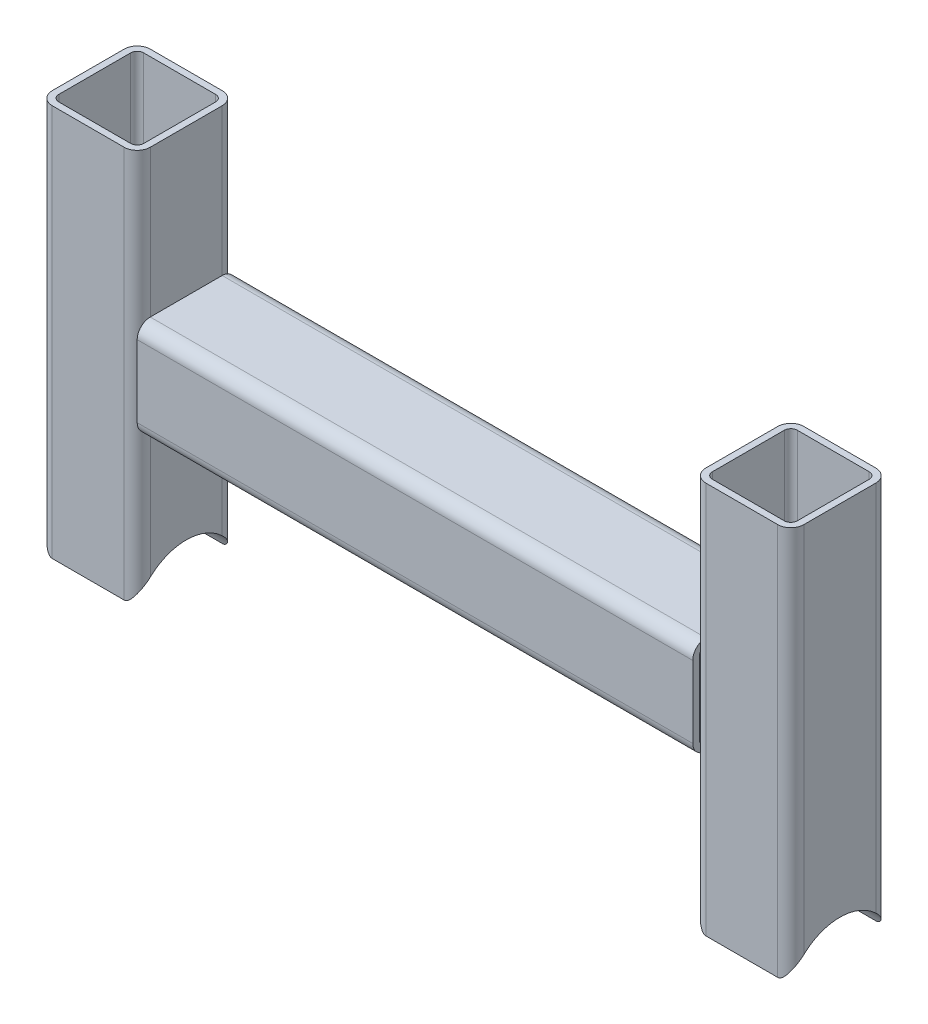
from build123d import *

# Parameters (mm, degrees)
GB_T_6728_2002_SQUARE_HOLLOW_SECTION_STE_DEPTH = 120
GB_T_6728_2002_SQUARE_HOLLOW_SECTION_2_DEPTH   = 120
GB_T_6728_2002_SQUARE_HOLLOW_SECTION_3_DEPTH   = 202
CUT_EXTRUDE1_DEPTH                             = 131.575648572
CUT_EXTRUDE1_DEPTH_BACK                        = 131.575648572
SKETCH3_R                                      = 16


with BuildPart() as part:
    # Sketch1 → Gb／t 6728—2002 Square hollow section steel 30×2-example.com(1) (new body)
    with BuildSketch(Plane(origin=(-100, -60, 0), x_dir=(-1, 0, 0), z_dir=(0, 1, 0))):
        with BuildLine():
            Line((-11, -15), (11, -15))
            ThreePointArc((11, -15), (13.828427125, -13.828427125), (15, -11))
            Line((15, -11), (15, 11))
            ThreePointArc((15, 11), (13.828427125, 13.828427125), (11, 15))
            Line((11, 15), (-11, 15))
            ThreePointArc((-11, 15), (-13.828427125, 13.828427125), (-15, 11))
            Line((-15, 11), (-15, -11))
            ThreePointArc((-15, -11), (-13.828427125, -13.828427125), (-11, -15))
        make_face()
        with BuildLine():
            Line((-11, -13), (11, -13))
            ThreePointArc((11, -13), (12.414213562, -12.414213562), (13, -11))
            Line((13, -11), (13, 11))
            ThreePointArc((13, 11), (12.414213562, 12.414213562), (11, 13))
            Line((11, 13), (-11, 13))
            ThreePointArc((-11, 13), (-12.414213562, 12.414213562), (-13, 11))
            Line((-13, 11), (-13, -11))
            ThreePointArc((-13, -11), (-12.414213562, -12.414213562), (-11, -13))
        make_face(mode=Mode.SUBTRACT)
    extrude(amount=GB_T_6728_2002_SQUARE_HOLLOW_SECTION_STE_DEPTH)


with BuildPart() as body_2:
    # Sketch1 on segment 2 (carried to segment 2) → Gb_t 6728_2002 Square hollow section 2 (new body)
    with BuildSketch(Plane(origin=(100, -60, 0), x_dir=(-1, 0, 0), z_dir=(0, 1, 0))):
        with BuildLine():
            Line((-11, -15), (11, -15))
            ThreePointArc((11, -15), (13.828427125, -13.828427125), (15, -11))
            Line((15, -11), (15, 11))
            ThreePointArc((15, 11), (13.828427125, 13.828427125), (11, 15))
            Line((11, 15), (-11, 15))
            ThreePointArc((-11, 15), (-13.828427125, 13.828427125), (-15, 11))
            Line((-15, 11), (-15, -11))
            ThreePointArc((-15, -11), (-13.828427125, -13.828427125), (-11, -15))
        make_face()
        with BuildLine():
            Line((-11, -13), (11, -13))
            ThreePointArc((11, -13), (12.414213562, -12.414213562), (13, -11))
            Line((13, -11), (13, 11))
            ThreePointArc((13, 11), (12.414213562, 12.414213562), (11, 13))
            Line((11, 13), (-11, 13))
            ThreePointArc((-11, 13), (-12.414213562, 12.414213562), (-13, 11))
            Line((-13, 11), (-13, -11))
            ThreePointArc((-13, -11), (-12.414213562, -12.414213562), (-11, -13))
        make_face(mode=Mode.SUBTRACT)
    extrude(amount=GB_T_6728_2002_SQUARE_HOLLOW_SECTION_2_DEPTH)


with BuildPart() as body_3:
    # Sketch1 on segment 3 (carried to segment 3) → Gb_t 6728_2002 Square hollow section 3 (new body)
    with BuildSketch(Plane(origin=(101, 0, 0), x_dir=(0, -1, 0), z_dir=(-1, 0, 0))):
        with BuildLine():
            Line((-11, -15), (11, -15))
            ThreePointArc((11, -15), (13.828427125, -13.828427125), (15, -11))
            Line((15, -11), (15, 11))
            ThreePointArc((15, 11), (13.828427125, 13.828427125), (11, 15))
            Line((11, 15), (-11, 15))
            ThreePointArc((-11, 15), (-13.828427125, 13.828427125), (-15, 11))
            Line((-15, 11), (-15, -11))
            ThreePointArc((-15, -11), (-13.828427125, -13.828427125), (-11, -15))
        make_face()
        with BuildLine():
            Line((-11, -13), (11, -13))
            ThreePointArc((11, -13), (12.414213562, -12.414213562), (13, -11))
            Line((13, -11), (13, 11))
            ThreePointArc((13, 11), (12.414213562, 12.414213562), (11, 13))
            Line((11, 13), (-11, 13))
            ThreePointArc((-11, 13), (-12.414213562, 12.414213562), (-13, 11))
            Line((-13, 11), (-13, -11))
            ThreePointArc((-13, -11), (-12.414213562, -12.414213562), (-11, -13))
        make_face(mode=Mode.SUBTRACT)
    extrude(amount=GB_T_6728_2002_SQUARE_HOLLOW_SECTION_3_DEPTH)

    # Gb_t 6728_2002 Square hollow section 3 e
    split(bisect_by=Plane(origin=(85, 0, 0), x_dir=(0, -1, 0), z_dir=(-1, 0, 0)), keep=Keep.TOP)

    # Gb_t 6728_2002 Square hollow section 4
    split(bisect_by=Plane.YZ.offset(-85), keep=Keep.TOP)


with BuildPart() as cut_extrude1_tool:
    # Sketch3 → Cut-Extrude1 (new, two sides: drawn at the far end of the back side and taken through both)
    with BuildSketch(Plane(origin=(0, 0, 0), x_dir=(0, 0, -1), z_dir=(1, 0, 0)).offset(-CUT_EXTRUDE1_DEPTH_BACK)):
        with Locations((0, -65.567764363)):
            Circle(SKETCH3_R)
    extrude(amount=CUT_EXTRUDE1_DEPTH + CUT_EXTRUDE1_DEPTH_BACK)


with BuildPart() as part_1:
    add(part.part)

    # Cut-Extrude1: cut by cut_extrude1_tool
    add(cut_extrude1_tool.part, mode=Mode.SUBTRACT)


with BuildPart() as body_2_1:
    add(body_2.part)

    # Cut-Extrude1: cut by cut_extrude1_tool
    add(cut_extrude1_tool.part, mode=Mode.SUBTRACT)


solid = Compound([body_3.part, part_1.part, body_2_1.part])
